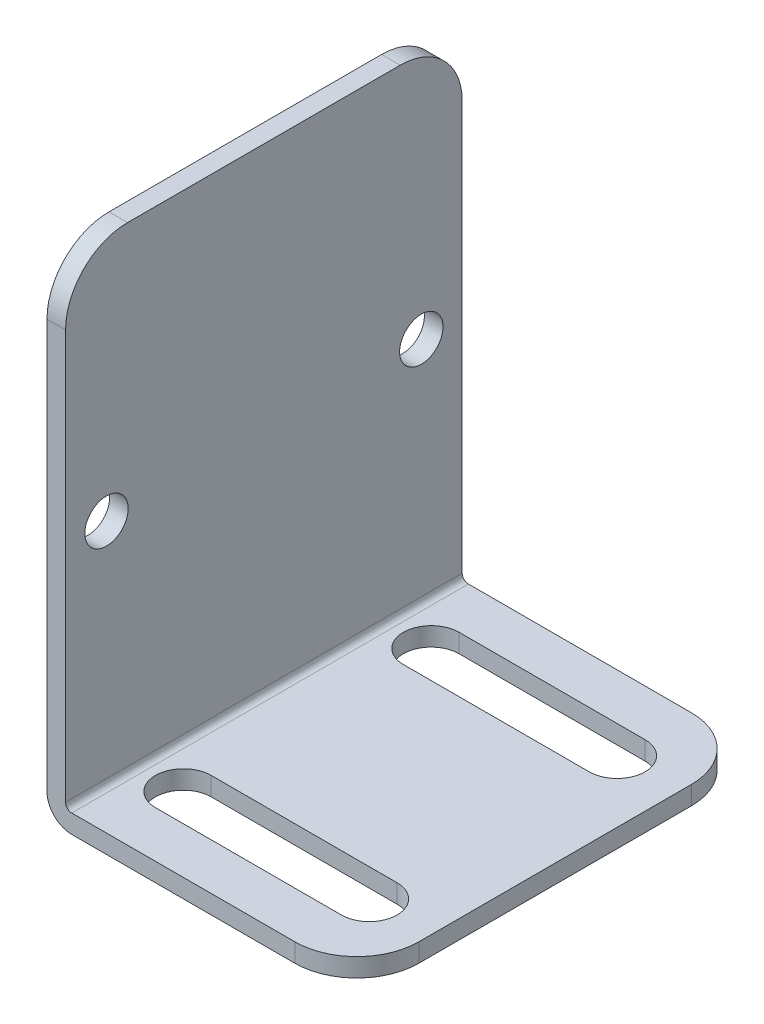
SolidWorks part; units mm, degrees
material "SUS304 T=1.5mm"
ref_plane "前视基准面" through (0, 0, 0) normal (0, 0, 1) x (1, 0, 0)
ref_plane "上视基准面" through (0, 0, 0) normal (0, 1, 0) x (1, 0, 0)
ref_plane "右视基准面" through (0, 0, 0) normal (1, 0, 0) x (0, 0, -1)
sketch "草图1" plane through (0, 0, 0) normal (0, 0, 1) x (1, 0, 0)
  line L0 (0, 0) -> (0, 40)
  line L1 (0, 0) -> (25, 0)
  dimension "D1" = 40
  dimension "D2" = 25
extrude "拉伸-薄壁1" add sketch "草图1" along normal blind 32 thin
fillet "圆角1" radius 0.5 1 edges at (1.5, 1.5, 16)
fillet "圆角2" radius 2 1 edges at (0, 0, 16)
fillet "圆角3" radius 5 4 edges at (25, 0.75, 32) (25, 0.75, 0) (0.75, 40, 0) (0.75, 40, 32)
sketch "草图2" plane through (0, 0, 0) normal (-1, 0, 0) x (0, 0, 1)
  line L0 (16, 40) -> (16, 15.6303) construction
  line L1 (27, 40) -> (5, 40) construction
  circle A0 centre (3.3, 20) radius 1.75
  circle A1 centre (28.7, 20) radius 1.75
  dimension "D1" = 25.4
  dimension "D2" = 3.5
  dimension "D3" = 20
extrude "切除-拉伸1" cut sketch "草图2" against normal up to next
sketch "草图3" plane through (0, 1.5, 0) normal (0, 1, 0) x (1, 0, 0)
  line L0 (5, -6) -> (20, -6) construction
  line L1 (5, -3.75) -> (20, -3.75)
  line L2 (5, -8.25) -> (20, -8.25)
  line L3 (5, -26) -> (20, -26) construction
  line L4 (5, -23.75) -> (20, -23.75)
  line L5 (5, -28.25) -> (20, -28.25)
  line L6 (25, -16) -> (6.0706, -16) construction
  line L7 (25, -27) -> (25, -5) construction
  arc A0 (5, -3.75) -> (5, -8.25) centre (5, -6) ccw
  arc A1 (20, -8.25) -> (20, -3.75) centre (20, -6) ccw
  arc A2 (5, -23.75) -> (5, -28.25) centre (5, -26) ccw
  arc A3 (20, -28.25) -> (20, -23.75) centre (20, -26) ccw
  point P2 (12.5, -6)
  point P7 (12.5, -26)
  dimension "D3" = 5
  dimension "D1" = 20
  dimension "D2" = 15
  dimension "D4" = 4.5
extrude "切除-拉伸2" cut sketch "草图3" against normal up to next
